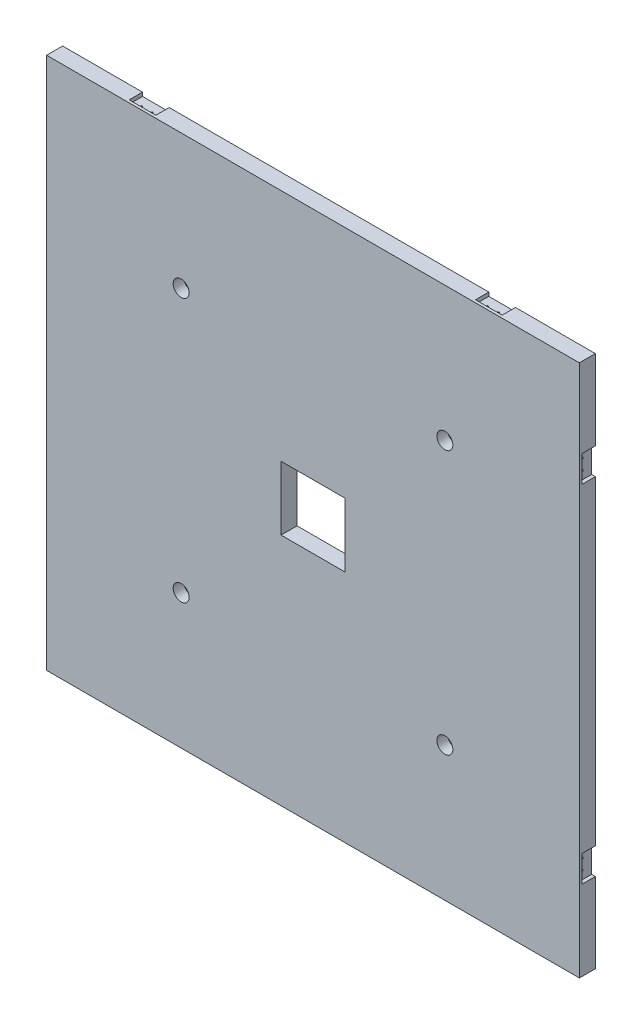
from build123d import *

# Parameters (mm, degrees)
SKETCH1_W                  = 1000
SKETCH1_H                  = 1000
SKETCH1_W_2                = 120
SKETCH1_H_2                = 120
BOSS_EXTRUDE1_DEPTH        = 30
SKETCH2_R                  = 15
CUT_EXTRUDE1_DEPTH         = 20
SKETCH3_W                  = 50
SKETCH3_H                  = 90
CUT_EXTRUDE2_DEPTH         = 7
CIRPATTERN1_COUNT          = 4
M4_TAPPED_HOLE1_AT_2_COUNT = 2
M4_TAPPED_HOLE1_AT_2_PITCH = 20
M4_TAPPED_HOLE1_AT_3_COUNT = 2
M4_TAPPED_HOLE1_AT_3_PITCH = 650
M4_TAPPED_HOLE1_AT_4_COUNT = 2
M4_TAPPED_HOLE1_AT_4_PITCH = 670
CIRPATTERN2_COUNT          = 4


with BuildPart() as part:
    # Sketch1 → Boss-Extrude1 (new body)
    with BuildSketch(Plane.XY):
        Rectangle(SKETCH1_W, SKETCH1_H)
        Rectangle(SKETCH1_W_2, SKETCH1_H_2, mode=Mode.SUBTRACT)
    extrude(amount=BOSS_EXTRUDE1_DEPTH)

    # Sketch2 → Cut-Extrude1 (cut)
    with BuildSketch(Plane.XY.offset(30)):
        with Locations((-247.487373415, 247.487373415)):
            Circle(SKETCH2_R)
        with Locations((247.487373415, 247.487373415)):
            Circle(SKETCH2_R)
        with Locations((247.487373415, -247.487373415)):
            Circle(SKETCH2_R)
        with Locations((-247.487373415, -247.487373415)):
            Circle(SKETCH2_R)
    extrude(amount=-CUT_EXTRUDE1_DEPTH, mode=Mode.SUBTRACT)

    # Sketch3 → Cut-Extrude2 (cut)
    with BuildSketch(Plane(origin=(0, 500, 0), x_dir=(1, 0, 0), z_dir=(0, 1, 0))):
        with Locations((-325, 20)):
            Rectangle(SKETCH3_W, SKETCH3_H)
        with Locations((325, 20)):
            Rectangle(SKETCH3_W, SKETCH3_H)
    cut_extrude2 = extrude(amount=-CUT_EXTRUDE2_DEPTH, mode=Mode.SUBTRACT)

    # CirPattern1: Cut-Extrude2 ×4 about axis
    cirpattern1_axis = Axis((0, 0, 0), (0, 0, 1))
    for i in range(1, CIRPATTERN1_COUNT):
        add(cut_extrude2.rotate(cirpattern1_axis, i * 360 / CIRPATTERN1_COUNT), mode=Mode.SUBTRACT)

    # Sketch6 → M4 Tapped Hole1 (revolve, cut)
    with BuildSketch(Plane(origin=(335, -493, 17.5), x_dir=(0, 0, -1), z_dir=(1, 0, 0))):
        Polygon((0, 0), (0, 11.091420021), (1.65, 10.1), (1.65, 0), align=None)
    m4_tapped_hole1 = revolve(axis=Axis((335, -499.35, 17.5), (0, 1, 0)), mode=Mode.SUBTRACT)

    # M4 Tapped Hole1 at 2: M4 Tapped Hole1 ×2
    with Locations(*[(-i * M4_TAPPED_HOLE1_AT_2_PITCH, 0, 0) for i in range(1, M4_TAPPED_HOLE1_AT_2_COUNT)]):
        add(m4_tapped_hole1, mode=Mode.SUBTRACT)

    # M4 Tapped Hole1 at 3: M4 Tapped Hole1 ×2
    with Locations(*[(-i * M4_TAPPED_HOLE1_AT_3_PITCH, 0, 0) for i in range(1, M4_TAPPED_HOLE1_AT_3_COUNT)]):
        add(m4_tapped_hole1, mode=Mode.SUBTRACT)

    # M4 Tapped Hole1 at 4: M4 Tapped Hole1 ×2
    with Locations(*[(-i * M4_TAPPED_HOLE1_AT_4_PITCH, 0, 0) for i in range(1, M4_TAPPED_HOLE1_AT_4_COUNT)]):
        add(m4_tapped_hole1, mode=Mode.SUBTRACT)

    # CirPattern2: M4 Tapped Hole1 ×4 about axis
    cirpattern2_axis = Axis((0, 0, 0), (0, 0, -1))
    for i in range(1, CIRPATTERN2_COUNT):
        add(m4_tapped_hole1.rotate(cirpattern2_axis, i * 360 / CIRPATTERN2_COUNT), mode=Mode.SUBTRACT)

    # CirPattern2 copy 1 sketch → CirPattern2 copy 1 (revolve, cut)
    with BuildSketch(Plane(origin=(-493, -315, 17.5), x_dir=(0, 0, -1), z_dir=(0, -1, 0))):
        Polygon((0, 0), (0, 11.091420021), (1.65, 10.1), (1.65, 0), align=None)
    revolve(axis=Axis((-499.35, -315, 17.5), (1, 0, 0)), mode=Mode.SUBTRACT)

    # CirPattern2 copy 2 sketch → CirPattern2 copy 2 (revolve, cut)
    with BuildSketch(Plane(origin=(-315, 493, 17.5), x_dir=(0, 0, -1), z_dir=(-1, 0, 0))):
        Polygon((0, 0), (0, 11.091420021), (1.65, 10.1), (1.65, 0), align=None)
    revolve(axis=Axis((-315, 499.35, 17.5), (0, -1, 0)), mode=Mode.SUBTRACT)

    # CirPattern2 copy 3 sketch → CirPattern2 copy 3 (revolve, cut)
    with BuildSketch(Plane(origin=(493, 315, 17.5), x_dir=(0, 0, -1), z_dir=(0, 1, 0))):
        Polygon((0, 0), (0, 11.091420021), (1.65, 10.1), (1.65, 0), align=None)
    revolve(axis=Axis((499.35, 315, 17.5), (-1, 0, 0)), mode=Mode.SUBTRACT)

    # CirPattern2 copy 4 sketch → CirPattern2 copy 4 (revolve, cut)
    with BuildSketch(Plane(origin=(-493, 315, 17.5), x_dir=(0, 0, -1), z_dir=(0, -1, 0))):
        Polygon((0, 0), (0, 11.091420021), (1.65, 10.1), (1.65, 0), align=None)
    revolve(axis=Axis((-499.35, 315, 17.5), (1, 0, 0)), mode=Mode.SUBTRACT)

    # CirPattern2 copy 5 sketch → CirPattern2 copy 5 (revolve, cut)
    with BuildSketch(Plane(origin=(315, 493, 17.5), x_dir=(0, 0, -1), z_dir=(-1, 0, 0))):
        Polygon((0, 0), (0, 11.091420021), (1.65, 10.1), (1.65, 0), align=None)
    revolve(axis=Axis((315, 499.35, 17.5), (0, -1, 0)), mode=Mode.SUBTRACT)

    # CirPattern2 copy 6 sketch → CirPattern2 copy 6 (revolve, cut)
    with BuildSketch(Plane(origin=(493, -315, 17.5), x_dir=(0, 0, -1), z_dir=(0, 1, 0))):
        Polygon((0, 0), (0, 11.091420021), (1.65, 10.1), (1.65, 0), align=None)
    revolve(axis=Axis((499.35, -315, 17.5), (-1, 0, 0)), mode=Mode.SUBTRACT)

    # CirPattern2 copy 7 sketch → CirPattern2 copy 7 (revolve, cut)
    with BuildSketch(Plane(origin=(-493, 335, 17.5), x_dir=(0, 0, -1), z_dir=(0, -1, 0))):
        Polygon((0, 0), (0, 11.091420021), (1.65, 10.1), (1.65, 0), align=None)
    revolve(axis=Axis((-499.35, 335, 17.5), (1, 0, 0)), mode=Mode.SUBTRACT)

    # CirPattern2 copy 8 sketch → CirPattern2 copy 8 (revolve, cut)
    with BuildSketch(Plane(origin=(335, 493, 17.5), x_dir=(0, 0, -1), z_dir=(-1, 0, 0))):
        Polygon((0, 0), (0, 11.091420021), (1.65, 10.1), (1.65, 0), align=None)
    revolve(axis=Axis((335, 499.35, 17.5), (0, -1, 0)), mode=Mode.SUBTRACT)

    # CirPattern2 copy 9 sketch → CirPattern2 copy 9 (revolve, cut)
    with BuildSketch(Plane(origin=(493, -335, 17.5), x_dir=(0, 0, -1), z_dir=(0, 1, 0))):
        Polygon((0, 0), (0, 11.091420021), (1.65, 10.1), (1.65, 0), align=None)
    revolve(axis=Axis((499.35, -335, 17.5), (-1, 0, 0)), mode=Mode.SUBTRACT)


solid = part.part
